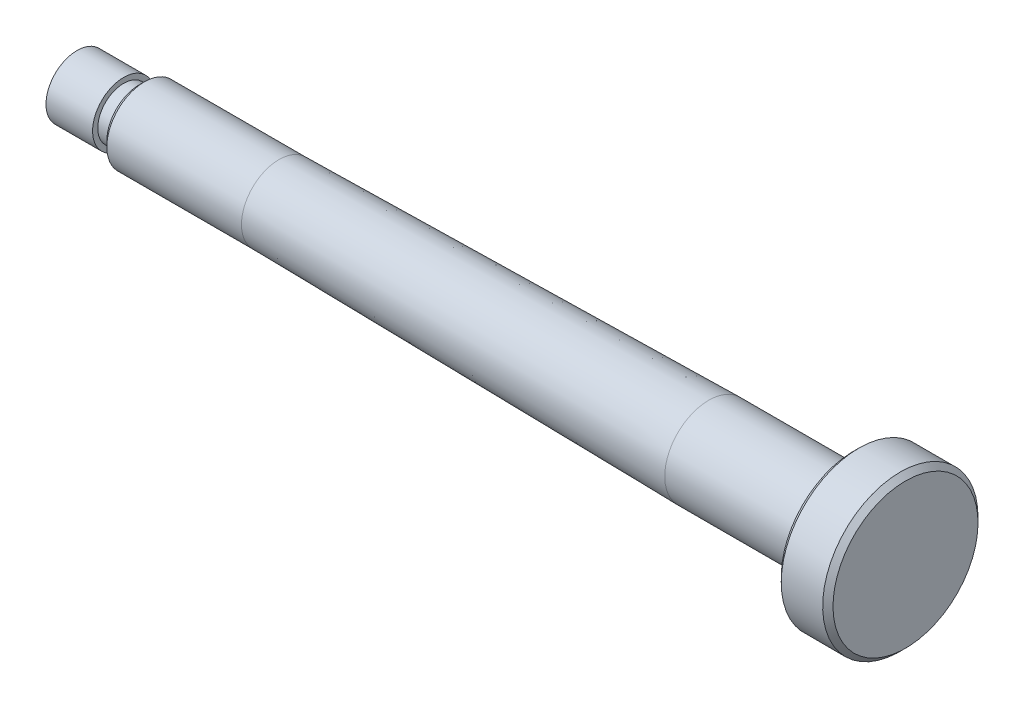
from build123d import *

# Parameters (mm, degrees)
CHAMFER_1_SIZE = 1


with BuildPart() as part:
    # 草图1 → 旋转1 (revolve)
    with BuildSketch(Plane.XY):
        Polygon((134.449619949, -49.868352239), (161.449619949, -49.868352239), (244.449619949, -48.618352239), (272.449619949, -48.618352239), (272.449619949, -42.118352239), (282.449619949, -42.118352239), (282.449619949, -57.118352239), (122.449619949, -57.118352239), (122.449619949, -51.118352239), (131.449619949, -51.118352239), (131.449619949, -52.118352239), (134.449619949, -52.118352239), align=None)
    revolve(axis=Axis((272.449619949, -57.118352239, 0), (-1, 0, 0)))

    # 倒角1
    chamfer_1_edges = [part.edges().sort_by_distance(p)[0] for p in [
        (282.449619949, -72.118352239, 0),
        (272.449619949, -72.118352239, 0),
        (134.449619949, -64.368352239, 0),
    ]]
    chamfer(chamfer_1_edges, length=CHAMFER_1_SIZE)


solid = part.part
